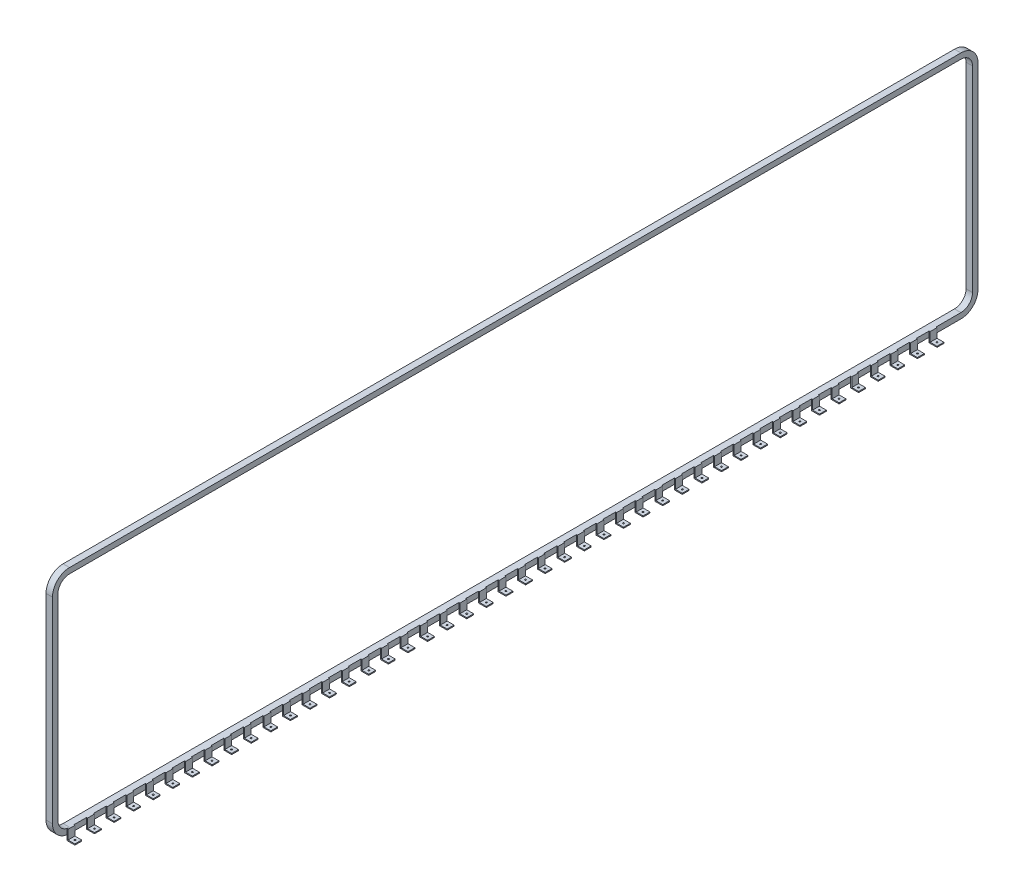
SolidWorks part; units mm, degrees
ref_plane "前视基准面" through (0, 0, 0) normal (0, 0, 1) x (1, 0, 0)
ref_plane "上视基准面" through (0, 0, 0) normal (0, 1, 0) x (1, 0, 0)
ref_plane "右视基准面" through (0, 0, 0) normal (1, 0, 0) x (0, 0, -1)
sketch "草图1" plane through (0, 0, 0) normal (1, 0, 0) x (0, 0, -1)
  line L1 (-1300, 320) -> (1300, 320)
  line L2 (-1333.81, 286.19) -> (-1333.81, -286.19)
  line L3 (-1300, -320) -> (1300, -320)
  line L4 (1333.81, 286.19) -> (1333.81, -286.19)
  line L5 (-1333.81, 320) -> (1333.81, -320) construction
  line L6 (-1333.81, -320) -> (1333.81, 320) construction
  arc A0 (-1300, 320) -> (-1333.81, 286.19) centre (-1300, 286.19) ccw
  arc A1 (-1333.81, -286.19) -> (-1300, -320) centre (-1300, -286.19) ccw
  arc A2 (1300, -320) -> (1333.81, -286.19) centre (1300, -286.19) ccw
  arc A3 (1333.81, 286.19) -> (1300, 320) centre (1300, 286.19) ccw
  point P0 (0, 0)
  dimension "D1" = 33.81
  dimension "D2" = 640
  dimension "D3" = 2600
extrude "拉伸-薄壁1" add sketch "草图1" along normal blind 18.8 thin thin type one direction wall 16
sketch "草图2" plane through (18.8, 0, 0) normal (1, 0, 0) x (0, 0, -1)
  line L0 (-1300, -320) -> (1300, -320) construction
  line L1 (-1307.35, -350) -> (-1287.35, -350)
  line L2 (-1307.35, -350) -> (-1307.35, -320)
  line L3 (-1307.35, -320) -> (-1287.35, -320)
  line L4 (-1287.35, -350) -> (-1287.35, -320)
  dimension "D1" = 20
  dimension "D2" = 30
  dimension "D3" = 7.35
extrude "凸台-拉伸1" add sketch "草图2" along normal blind 3 contours L1 L4 L3 L2
sketch "草图3" plane through (21.8, 0, 0) normal (1, 0, 0) x (0, 0, -1)
  line L0 (-1287.35, -350) -> (-1287.35, -320) construction
  line L1 (-1307.35, -350) -> (-1287.35, -350)
  line L2 (-1307.35, -350) -> (-1307.35, -347)
  line L3 (-1307.35, -347) -> (-1287.35, -347)
  line L4 (-1287.35, -350) -> (-1287.35, -347)
  dimension "D1" = 3
extrude "凸台-拉伸2" add sketch "草图3" along normal blind 20
hole_wizard "M5 螺纹孔1" positions "草图4" profile "草图5" tap size "M5" standard "GB" end condition through all
sketch "草图4" plane through (0, -350, 0) normal (0, -1, 0) x (-1, 0, 0)
  line L0 (-41.8, -1297.35) -> (-25.5961, -1297.35) construction
  line L1 (-41.8, -1307.35) -> (-41.8, -1287.35) construction
  point P0 (-31.8, -1297.35)
  dimension "D1" = 10
sketch "草图5" plane through (31.8, -350, 1297.35) normal (1, 0, 0) x (0, 0, -1)
  line L0 (0, 0) -> (0, 686)
  line L1 (0, 686) -> (2.1, 686)
  line L2 (2.1, 686) -> (2.1, 0)
  line L5 (2.1, 0) -> (0, 0)
  line L11 (0, -6.35) -> (0, 107.95) construction
  dimension "通孔螺纹孔钻头直径" = 4.2
  dimension "通孔螺纹孔钻头深度" = 686
cosmetic thread "孔螺蚊线1" parameters "D2"=5
pattern_linear "阵列(线性)1" count 45 spacing 57.15 along (0, 0, -1) of "M5 螺纹孔1", "凸台-拉伸2", "凸台-拉伸1"
